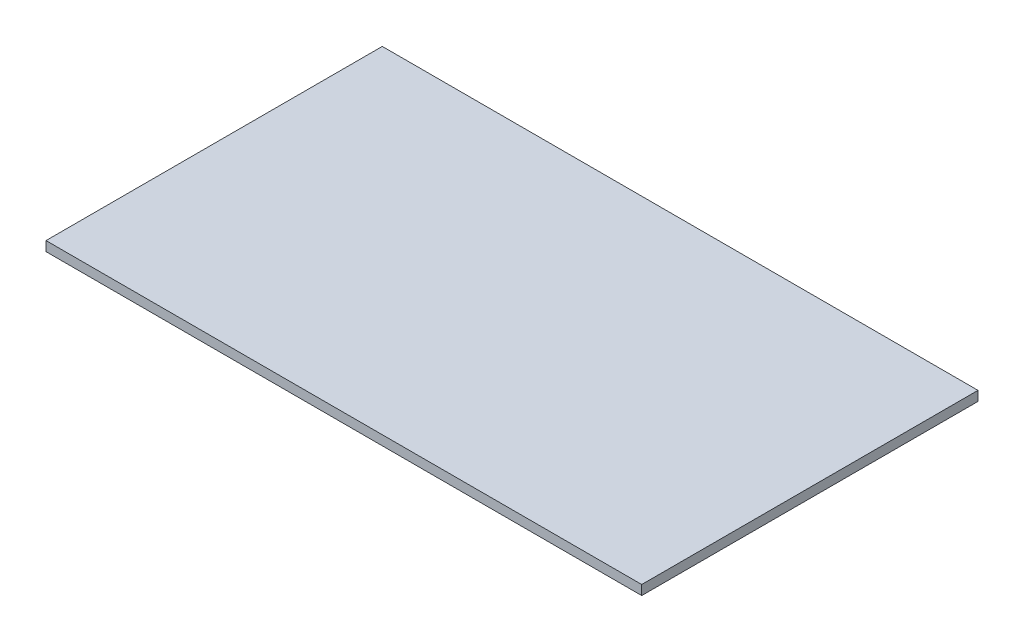
SolidWorks part; units mm, degrees
ref_plane "Front Plane" through (0, 0, 0) normal (0, 0, 1) x (1, 0, 0)
ref_plane "Top Plane" through (0, 0, 0) normal (0, 1, 0) x (1, 0, 0)
ref_plane "Right Plane" through (0, 0, 0) normal (1, 0, 0) x (0, 0, -1)
sketch "Sketch1" plane through (0, 0, 0) normal (0, 1, 0) x (1, 0, 0)
  line L1 (-3400, 2400) -> (3400, 2400)
  line L2 (-3400, 2400) -> (-3400, -2400)
  line L3 (-3400, -2400) -> (3400, -2400)
  line L4 (3400, 2400) -> (3400, -2400)
  line L5 (-3400, 2400) -> (3400, -2400) construction
  line L6 (-3400, -2400) -> (3400, 2400) construction
  point P0 (0, 0)
  dimension "D1" = 6800
  dimension "D2" = 4800
extrude "Boss-Extrude1" add sketch "Sketch1" along normal blind 100
sketch "Sketch2" plane through (0, 100, 0) normal (0, 1, 0) x (1, 0, 0)
  line L1 (-3400, 2400) -> (2800, 2400)
  line L2 (-3400, 2400) -> (-3400, -1100)
  line L3 (-3400, -1100) -> (2800, -1100)
  line L4 (2800, 2400) -> (2800, -1100)
  dimension "D1" = 3500
  dimension "D2" = 6200
extrude "Cut-Extrude1" cut sketch "Sketch2" against normal through all flip side to cut
